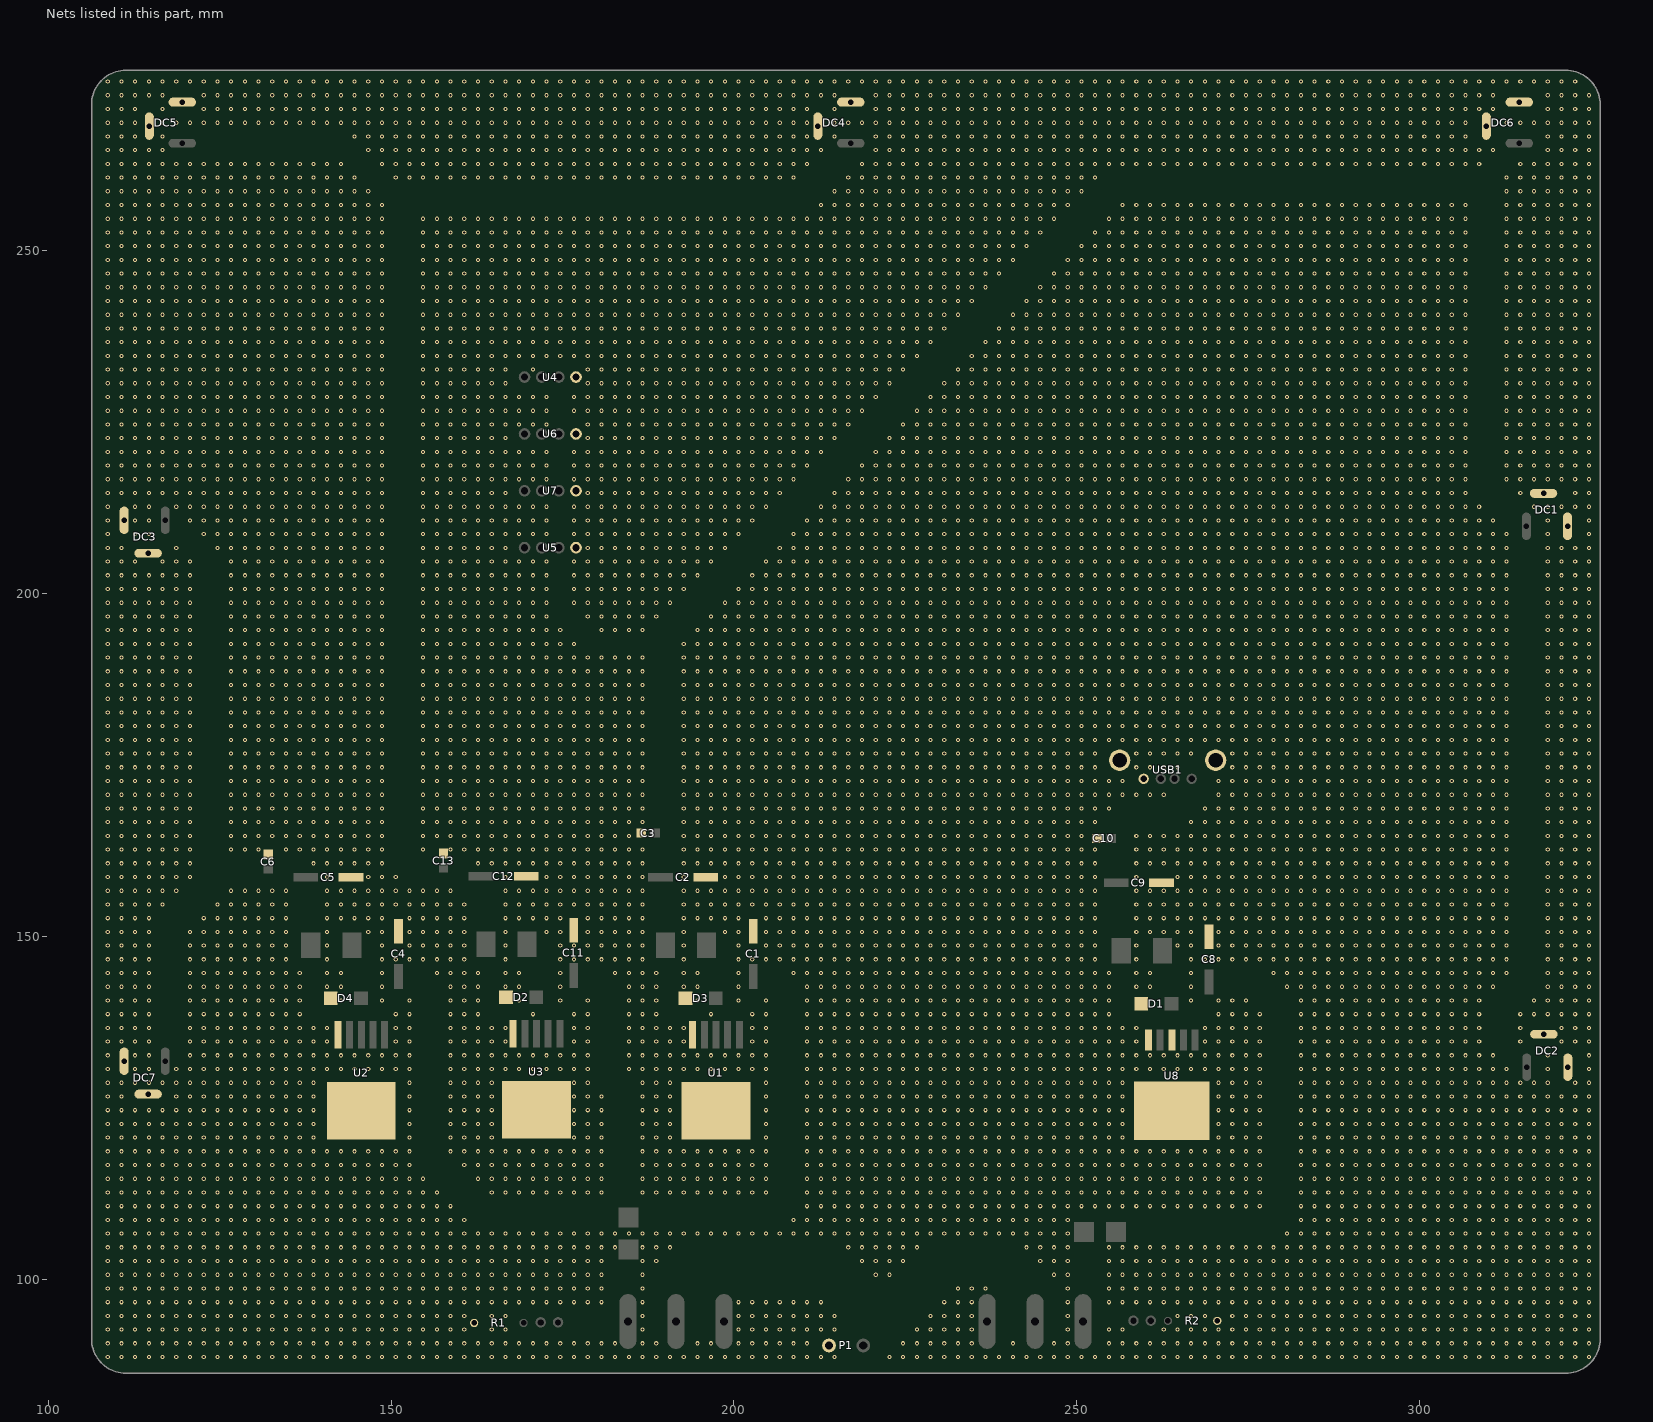
[diagram p0: the nets of this part, all layers, seen from the top]
# Altium PCB MISC49942.pcbdoc (part 3 of 4)
Units mm, origin at the board's own origin, x right, y up, seen from the top; angles counter-clockwise.
Board outline 220 x 190 mm, 2 copper layers (Top Layer, Bottom Layer), stack 1.58 mm thick; 45 components, 14 nets, 127 pads, 8689 vias.

## Via types
v1: diameter 0.61, hole 0.305, Top Layer to Bottom Layer, 8689 vias

## Nets (pads, with @x,y where several pads share a name; then routed paths per layer and width w, separated by ;. In a path a pad name is that pad's centre, name@x,y a point inside that pad or via, vN(x,y) a via of type N, cw(c..) or ccw(c..) an arc to the next point about the centre after c; other vN are vias at no path point) (continued)
GND: (continued)
  other v1: 270.684,158.669 272.684,158.669 274.684,158.669 276.684,158.669 278.684,158.669 280.684,158.669 282.684,158.669 284.684,158.669 286.684,158.669 288.684,158.669 290.684,158.669 292.684,158.669 294.684,158.669 296.684,158.669 298.684,158.669 300.684,158.669 302.684,158.669 304.684,158.669 306.684,158.669 308.684,158.669 310.684,158.669 312.684,158.669 318.684,158.669 320.684,158.669 322.684,158.669 324.684,158.669 108.684,160.669 110.684,160.669 112.684,160.669 114.684,160.669 116.684,160.669 118.684,160.669 120.684,160.669 138.684,160.669 140.684,160.669 142.684,160.669 144.684,160.669 146.684,160.669 148.684,160.669 162.684,160.669 164.684,160.669 166.684,160.669 168.684,160.669 170.684,160.669 172.684,160.669 174.684,160.669 176.684,160.669 178.684,160.669 180.684,160.669 182.684,160.669 184.684,160.669 186.684,160.669 192.684,160.669 194.684,160.669 196.684,160.669 198.684,160.669 200.684,160.669 202.684,160.669 204.684,160.669 206.684,160.669 208.684,160.669 210.684,160.669 212.684,160.669 214.684,160.669 216.684,160.669 218.684,160.669 220.684,160.669 222.684,160.669 224.684,160.669 226.684,160.669 228.684,160.669 230.684,160.669 232.684,160.669 234.684,160.669 236.684,160.669 238.684,160.669 240.684,160.669 242.684,160.669 244.684,160.669 246.684,160.669 248.684,160.669 250.684,160.669 252.684,160.669 258.684,160.669 260.684,160.669 262.684,160.669 264.684,160.669 266.684,160.669 268.684,160.669 270.684,160.669 272.684,160.669 274.684,160.669 276.684,160.669 278.684,160.669 280.684,160.669 282.684,160.669 284.684,160.669 286.684,160.669 288.684,160.669 290.684,160.669 292.684,160.669 294.684,160.669 296.684,160.669 298.684,160.669 300.684,160.669 302.684,160.669 304.684,160.669 306.684,160.669 308.684,160.669 310.684,160.669 312.684,160.669 318.684,160.669 320.684,160.669 322.684,160.669 324.684,160.669 108.684,162.669 110.684,162.669 112.684,162.669 114.684,162.669 116.684,162.669 118.684,162.669 120.684,162.669 126.684,162.669 128.684,162.669 130.684,162.669 134.684,162.669 136.684,162.669 138.684,162.669 140.684,162.669 142.684,162.669 144.684,162.669 146.684,162.669 148.684,162.669 154.684,162.669 158.684,162.669 160.684,162.669 162.684,162.669 164.684,162.669 166.684,162.669 168.684,162.669 170.684,162.669 172.684,162.669 174.684,162.669 176.684,162.669 178.684,162.669 180.684,162.669 182.684,162.669 184.684,162.669 186.684,162.669 192.684,162.669 194.684,162.669 196.684,162.669 198.684,162.669 200.684,162.669 202.684,162.669 204.684,162.669 206.684,162.669 208.684,162.669 210.684,162.669 212.684,162.669 214.684,162.669 216.684,162.669 218.684,162.669 220.684,162.669 222.684,162.669 224.684,162.669 226.684,162.669 228.684,162.669 230.684,162.669 232.684,162.669 234.684,162.669 236.684,162.669 238.684,162.669 240.684,162.669 242.684,162.669 244.684,162.669 246.684,162.669 248.684,162.669 250.684,162.669 252.684,162.669 258.684,162.669 260.684,162.669 262.684,162.669 264.684,162.669 266.684,162.669 268.684,162.669 270.684,162.669 272.684,162.669 274.684,162.669 276.684,162.669 278.684,162.669 280.684,162.669 282.684,162.669 284.684,162.669 286.684,162.669 288.684,162.669 290.684,162.669 292.684,162.669 294.684,162.669 296.684,162.669 298.684,162.669 300.684,162.669 302.684,162.669 304.684,162.669 306.684,162.669 308.684,162.669 310.684,162.669 312.684,162.669 318.684,162.669 320.684,162.669 322.684,162.669 324.684,162.669 108.684,164.669 110.684,164.669 112.684,164.669 114.684,164.669 116.684,164.669 118.684,164.669 120.684,164.669 126.684,164.669 128.684,164.669 130.684,164.669 132.684,164.669 134.684,164.669 136.684,164.669 138.684,164.669 140.684,164.669 142.684,164.669 144.684,164.669 146.684,164.669 148.684,164.669 154.684,164.669 156.684,164.669 158.684,164.669 160.684,164.669 162.684,164.669 164.684,164.669 166.684,164.669 168.684,164.669 170.684,164.669 172.684,164.669 174.684,164.669 176.684,164.669 178.684,164.669 180.684,164.669 182.684,164.669 184.684,164.669 192.684,164.669 194.684,164.669 196.684,164.669 198.684,164.669 200.684,164.669 202.684,164.669 204.684,164.669 206.684,164.669 208.684,164.669 210.684,164.669 212.684,164.669 214.684,164.669 216.684,164.669 218.684,164.669 220.684,164.669 222.684,164.669 224.684,164.669 226.684,164.669 228.684,164.669 230.684,164.669 232.684,164.669 234.684,164.669 236.684,164.669 238.684,164.669 240.684,164.669 242.684,164.669 244.684,164.669 246.684,164.669 248.684,164.669 250.684,164.669 258.684,164.669 260.684,164.669 262.684,164.669 264.684,164.669 266.684,164.669 268.684,164.669 270.684,164.669 272.684,164.669 274.684,164.669 276.684,164.669 278.684,164.669 280.684,164.669 282.684,164.669 284.684,164.669 286.684,164.669 288.684,164.669 290.684,164.669 292.684,164.669 294.684,164.669 296.684,164.669 298.684,164.669 300.684,164.669 302.684,164.669 304.684,164.669 306.684,164.669 308.684,164.669 310.684,164.669 312.684,164.669 318.684,164.669 320.684,164.669 322.684,164.669 324.684,164.669 108.684,166.669 110.684,166.669 112.684,166.669 114.684,166.669 116.684,166.669 118.684,166.669 120.684,166.669 126.684,166.669 128.684,166.669 130.684,166.669 132.684,166.669 134.684,166.669 136.684,166.669 138.684,166.669 140.684,166.669 142.684,166.669 144.684,166.669 146.684,166.669 148.684,166.669 154.684,166.669 156.684,166.669 158.684,166.669 160.684,166.669 162.684,166.669 164.684,166.669 166.684,166.669 168.684,166.669 170.684,166.669 172.684,166.669 174.684,166.669 176.684,166.669 178.684,166.669 180.684,166.669 182.684,166.669 184.684,166.669 186.684,166.669 192.684,166.669 194.684,166.669 196.684,166.669 198.684,166.669 200.684,166.669 202.684,166.669 204.684,166.669 206.684,166.669 208.684,166.669 210.684,166.669 212.684,166.669 214.684,166.669 216.684,166.669 218.684,166.669 220.684,166.669 222.684,166.669 224.684,166.669 226.684,166.669 228.684,166.669 230.684,166.669 232.684,166.669 234.684,166.669 236.684,166.669 238.684,166.669 240.684,166.669 242.684,166.669 244.684,166.669 246.684,166.669 248.684,166.669 250.684,166.669 252.684,166.669 266.684,166.669 268.684,166.669 270.684,166.669 272.684,166.669 274.684,166.669 276.684,166.669 278.684,166.669 280.684,166.669 282.684,166.669 284.684,166.669 286.684,166.669 288.684,166.669 290.684,166.669 292.684,166.669 294.684,166.669 296.684,166.669 298.684,166.669 300.684,166.669 302.684,166.669 304.684,166.669 306.684,166.669 308.684,166.669 310.684,166.669 312.684,166.669 318.684,166.669 320.684,166.669 322.684,166.669 324.684,166.669 108.684,168.669 110.684,168.669 112.684,168.669 114.684,168.669 116.684,168.669 118.684,168.669 120.684,168.669 126.684,168.669 128.684,168.669 130.684,168.669 132.684,168.669 134.684,168.669 136.684,168.669 138.684,168.669 140.684,168.669 142.684,168.669 144.684,168.669 146.684,168.669 148.684,168.669 154.684,168.669 156.684,168.669 158.684,168.669 160.684,168.669 162.684,168.669 164.684,168.669 166.684,168.669 168.684,168.669 170.684,168.669 172.684,168.669 174.684,168.669 176.684,168.669 178.684,168.669 180.684,168.669 182.684,168.669 184.684,168.669 186.684,168.669 192.684,168.669 194.684,168.669 196.684,168.669 198.684,168.669 200.684,168.669 202.684,168.669 204.684,168.669 206.684,168.669 208.684,168.669 210.684,168.669 212.684,168.669 214.684,168.669 216.684,168.669 218.684,168.669 220.684,168.669 222.684,168.669 224.684,168.669 226.684,168.669 228.684,168.669 230.684,168.669 232.684,168.669 234.684,168.669 236.684,168.669 238.684,168.669 240.684,168.669 242.684,168.669 244.684,168.669 246.684,168.669 248.684,168.669 250.684,168.669 252.684,168.669 254.684,168.669 268.684,168.669 270.684,168.669 272.684,168.669 274.684,168.669 276.684,168.669 278.684,168.669 280.684,168.669 282.684,168.669 284.684,168.669 286.684,168.669 288.684,168.669 290.684,168.669 292.684,168.669 294.684,168.669 296.684,168.669 298.684,168.669 300.684,168.669 302.684,168.669 304.684,168.669 306.684,168.669 308.684,168.669 310.684,168.669 312.684,168.669 318.684,168.669 320.684,168.669 322.684,168.669 324.684,168.669 108.684,170.669 110.684,170.669 112.684,170.669 114.684,170.669 116.684,170.669 118.684,170.669 120.684,170.669 126.684,170.669 128.684,170.669 130.684,170.669 132.684,170.669 134.684,170.669 136.684,170.669 138.684,170.669 140.684,170.669 142.684,170.669 144.684,170.669 146.684,170.669 148.684,170.669 154.684,170.669 156.684,170.669 158.684,170.669 160.684,170.669 162.684,170.669 164.684,170.669 166.684,170.669 168.684,170.669 170.684,170.669 172.684,170.669 174.684,170.669 176.684,170.669 178.684,170.669 180.684,170.669 182.684,170.669 184.684,170.669 186.684,170.669 192.684,170.669 194.684,170.669 196.684,170.669 198.684,170.669 200.684,170.669 202.684,170.669 204.684,170.669 206.684,170.669 208.684,170.669 210.684,170.669 212.684,170.669 214.684,170.669 216.684,170.669 218.684,170.669 220.684,170.669 222.684,170.669 224.684,170.669 226.684,170.669 228.684,170.669 230.684,170.669 232.684,170.669 234.684,170.669 236.684,170.669 238.684,170.669 240.684,170.669 242.684,170.669 244.684,170.669 246.684,170.669 248.684,170.669 250.684,170.669 252.684,170.669 254.684,170.669 256.684,170.669 258.684,170.669 260.684,170.669 262.684,170.669 270.684,170.669 272.684,170.669 274.684,170.669 276.684,170.669 278.684,170.669 280.684,170.669 282.684,170.669 284.684,170.669 286.684,170.669 288.684,170.669 290.684,170.669 292.684,170.669 294.684,170.669 296.684,170.669 298.684,170.669 300.684,170.669 302.684,170.669 304.684,170.669 306.684,170.669 308.684,170.669 310.684,170.669 312.684,170.669 318.684,170.669 320.684,170.669 322.684,170.669 324.684,170.669 108.684,172.669 110.684,172.669 112.684,172.669 114.684,172.669 116.684,172.669 118.684,172.669 120.684,172.669 126.684,172.669 128.684,172.669 130.684,172.669 132.684,172.669 134.684,172.669 136.684,172.669 138.684,172.669 140.684,172.669 142.684,172.669 144.684,172.669 146.684,172.669 148.684,172.669 154.684,172.669 156.684,172.669 158.684,172.669 160.684,172.669 162.684,172.669 164.684,172.669 166.684,172.669 168.684,172.669 170.684,172.669 172.684,172.669 174.684,172.669 176.684,172.669 178.684,172.669 180.684,172.669 182.684,172.669 184.684,172.669 186.684,172.669 192.684,172.669 194.684,172.669 196.684,172.669 198.684,172.669 200.684,172.669 202.684,172.669 204.684,172.669 206.684,172.669 208.684,172.669 210.684,172.669 212.684,172.669 214.684,172.669 216.684,172.669 218.684,172.669 220.684,172.669 222.684,172.669 224.684,172.669 226.684,172.669 228.684,172.669 230.684,172.669 232.684,172.669 234.684,172.669 236.684,172.669 238.684,172.669 240.684,172.669 242.684,172.669 244.684,172.669 246.684,172.669 248.684,172.669 250.684,172.669 252.684,172.669 254.684,172.669 256.684,172.669 270.684,172.669 272.684,172.669 274.684,172.669 276.684,172.669 278.684,172.669 280.684,172.669 282.684,172.669 284.684,172.669 286.684,172.669 288.684,172.669 290.684,172.669 292.684,172.669 294.684,172.669 296.684,172.669 298.684,172.669 300.684,172.669 302.684,172.669 304.684,172.669 306.684,172.669 308.684,172.669 310.684,172.669 312.684,172.669 318.684,172.669 320.684,172.669 322.684,172.669 324.684,172.669 108.684,174.669 110.684,174.669 112.684,174.669 114.684,174.669 116.684,174.669 118.684,174.669 120.684,174.669 126.684,174.669 128.684,174.669 130.684,174.669 132.684,174.669 134.684,174.669 136.684,174.669 138.684,174.669 140.684,174.669 142.684,174.669 144.684,174.669 146.684,174.669 148.684,174.669 154.684,174.669 156.684,174.669 158.684,174.669 160.684,174.669 162.684,174.669 164.684,174.669 166.684,174.669 168.684,174.669 170.684,174.669 172.684,174.669 174.684,174.669 176.684,174.669 178.684,174.669 180.684,174.669 182.684,174.669 184.684,174.669 186.684,174.669 192.684,174.669 194.684,174.669 196.684,174.669 198.684,174.669 200.684,174.669 202.684,174.669 204.684,174.669 206.684,174.669 208.684,174.669 210.684,174.669 212.684,174.669 214.684,174.669 216.684,174.669 218.684,174.669 220.684,174.669 222.684,174.669 224.684,174.669 226.684,174.669 228.684,174.669 230.684,174.669 232.684,174.669 234.684,174.669 236.684,174.669 238.684,174.669 240.684,174.669 242.684,174.669 244.684,174.669 246.684,174.669 248.684,174.669 250.684,174.669 252.684,174.669 258.684,174.669 260.684,174.669 262.684,174.669 264.684,174.669 272.684,174.669 274.684,174.669 276.684,174.669 278.684,174.669 280.684,174.669 282.684,174.669 284.684,174.669 286.684,174.669 288.684,174.669 290.684,174.669 292.684,174.669 294.684,174.669 296.684,174.669 298.684,174.669 300.684,174.669 302.684,174.669 304.684,174.669 306.684,174.669 308.684,174.669 310.684,174.669 312.684,174.669 318.684,174.669 320.684,174.669 322.684,174.669 324.684,174.669 108.684,176.669 110.684,176.669 112.684,176.669 114.684,176.669 116.684,176.669 118.684,176.669 120.684,176.669 126.684,176.669 128.684,176.669 130.684,176.669 132.684,176.669 134.684,176.669 136.684,176.669 138.684,176.669 140.684,176.669 142.684,176.669 144.684,176.669 146.684,176.669 148.684,176.669 154.684,176.669 156.684,176.669 158.684,176.669 160.684,176.669 162.684,176.669 164.684,176.669 166.684,176.669 168.684,176.669 170.684,176.669 172.684,176.669 174.684,176.669 176.684,176.669 178.684,176.669 180.684,176.669 182.684,176.669 184.684,176.669 186.684,176.669 192.684,176.669 194.684,176.669 196.684,176.669 198.684,176.669 200.684,176.669 202.684,176.669 204.684,176.669 206.684,176.669 208.684,176.669 210.684,176.669 212.684,176.669 214.684,176.669 216.684,176.669 218.684,176.669 220.684,176.669 222.684,176.669 224.684,176.669 226.684,176.669 228.684,176.669 230.684,176.669 232.684,176.669 234.684,176.669 236.684,176.669 238.684,176.669 240.684,176.669 242.684,176.669 244.684,176.669 246.684,176.669 248.684,176.669 250.684,176.669 252.684,176.669 258.684,176.669 260.684,176.669 262.684,176.669 264.684,176.669 266.684,176.669 272.684,176.669 274.684,176.669 276.684,176.669 278.684,176.669 280.684,176.669 282.684,176.669 284.684,176.669 286.684,176.669 288.684,176.669 290.684,176.669 292.684,176.669 294.684,176.669 296.684,176.669 298.684,176.669 300.684,176.669 302.684,176.669 304.684,176.669 306.684,176.669 308.684,176.669 310.684,176.669 312.684,176.669 318.684,176.669 320.684,176.669 322.684,176.669 324.684,176.669 108.684,178.669 110.684,178.669 112.684,178.669 114.684,178.669 116.684,178.669 118.684,178.669 120.684,178.669 126.684,178.669 128.684,178.669 130.684,178.669 132.684,178.669 134.684,178.669 136.684,178.669 138.684,178.669 140.684,178.669 142.684,178.669 144.684,178.669 146.684,178.669 148.684,178.669 154.684,178.669 156.684,178.669 158.684,178.669 160.684,178.669 162.684,178.669 164.684,178.669 166.684,178.669 168.684,178.669 170.684,178.669 172.684,178.669 174.684,178.669 176.684,178.669 178.684,178.669 180.684,178.669 182.684,178.669 184.684,178.669 186.684,178.669 192.684,178.669 194.684,178.669 196.684,178.669 198.684,178.669 200.684,178.669 202.684,178.669 204.684,178.669 206.684,178.669 208.684,178.669 210.684,178.669 212.684,178.669 214.684,178.669 216.684,178.669 218.684,178.669 220.684,178.669 222.684,178.669 224.684,178.669 226.684,178.669 228.684,178.669 230.684,178.669 232.684,178.669 234.684,178.669 236.684,178.669 238.684,178.669 240.684,178.669 242.684,178.669 244.684,178.669 246.684,178.669 248.684,178.669 250.684,178.669 252.684,178.669 254.684,178.669 256.684,178.669 258.684,178.669 260.684,178.669 262.684,178.669 264.684,178.669 266.684,178.669 268.684,178.669 270.684,178.669 272.684,178.669 274.684,178.669 276.684,178.669 278.684,178.669 280.684,178.669 282.684,178.669 284.684,178.669 286.684,178.669 288.684,178.669 290.684,178.669 292.684,178.669 294.684,178.669 296.684,178.669 298.684,178.669 300.684,178.669 302.684,178.669 304.684,178.669 306.684,178.669 308.684,178.669 310.684,178.669 312.684,178.669 318.684,178.669 320.684,178.669 322.684,178.669 324.684,178.669 108.684,180.669 110.684,180.669 112.684,180.669 114.684,180.669 116.684,180.669 118.684,180.669 120.684,180.669 126.684,180.669 128.684,180.669 130.684,180.669 132.684,180.669 134.684,180.669 136.684,180.669 138.684,180.669 140.684,180.669 142.684,180.669 144.684,180.669 146.684,180.669 148.684,180.669 154.684,180.669 156.684,180.669 158.684,180.669 160.684,180.669 162.684,180.669 164.684,180.669 166.684,180.669 168.684,180.669 170.684,180.669 172.684,180.669 174.684,180.669 176.684,180.669 178.684,180.669 180.684,180.669 182.684,180.669 184.684,180.669 186.684,180.669 192.684,180.669 194.684,180.669 196.684,180.669 198.684,180.669 200.684,180.669 202.684,180.669 204.684,180.669 206.684,180.669 208.684,180.669 210.684,180.669 212.684,180.669 214.684,180.669 216.684,180.669 218.684,180.669 220.684,180.669 222.684,180.669 224.684,180.669 226.684,180.669 228.684,180.669 230.684,180.669 232.684,180.669 234.684,180.669 236.684,180.669 238.684,180.669 240.684,180.669 242.684,180.669 244.684,180.669 246.684,180.669 248.684,180.669 250.684,180.669 252.684,180.669 254.684,180.669 256.684,180.669 258.684,180.669 260.684,180.669 262.684,180.669 264.684,180.669 266.684,180.669 268.684,180.669 270.684,180.669 272.684,180.669 274.684,180.669 276.684,180.669 278.684,180.669 280.684,180.669 282.684,180.669 284.684,180.669 286.684,180.669 288.684,180.669 290.684,180.669 292.684,180.669 294.684,180.669 296.684,180.669 298.684,180.669 300.684,180.669 302.684,180.669 304.684,180.669 306.684,180.669 308.684,180.669 310.684,180.669 312.684,180.669 318.684,180.669 320.684,180.669 322.684,180.669 324.684,180.669 108.684,182.669 110.684,182.669 112.684,182.669 114.684,182.669 116.684,182.669 118.684,182.669 120.684,182.669 126.684,182.669 128.684,182.669 130.684,182.669 132.684,182.669 134.684,182.669 136.684,182.669 138.684,182.669 140.684,182.669 142.684,182.669 144.684,182.669 146.684,182.669 148.684,182.669 154.684,182.669 156.684,182.669 158.684,182.669 160.684,182.669 162.684,182.669 164.684,182.669 166.684,182.669 168.684,182.669 170.684,182.669 172.684,182.669 174.684,182.669 176.684,182.669 178.684,182.669 180.684,182.669 182.684,182.669 184.684,182.669 186.684,182.669 192.684,182.669 194.684,182.669 196.684,182.669 198.684,182.669 200.684,182.669 202.684,182.669 204.684,182.669 206.684,182.669 208.684,182.669 210.684,182.669 212.684,182.669 214.684,182.669 216.684,182.669 218.684,182.669 220.684,182.669 222.684,182.669 224.684,182.669 226.684,182.669 228.684,182.669 230.684,182.669 232.684,182.669 234.684,182.669 236.684,182.669 238.684,182.669 240.684,182.669 242.684,182.669 244.684,182.669 246.684,182.669 248.684,182.669 250.684,182.669 252.684,182.669 254.684,182.669 256.684,182.669 258.684,182.669 260.684,182.669 262.684,182.669 264.684,182.669 266.684,182.669 268.684,182.669 270.684,182.669 272.684,182.669 274.684,182.669 276.684,182.669 278.684,182.669 280.684,182.669 282.684,182.669 284.684,182.669 286.684,182.669 288.684,182.669 290.684,182.669 292.684,182.669 294.684,182.669 296.684,182.669 298.684,182.669 300.684,182.669 302.684,182.669 304.684,182.669 306.684,182.669 308.684,182.669 310.684,182.669 312.684,182.669 318.684,182.669 320.684,182.669 322.684,182.669 324.684,182.669 108.684,184.669 110.684,184.669 112.684,184.669 114.684,184.669 116.684,184.669 118.684,184.669 120.684,184.669 126.684,184.669 128.684,184.669 130.684,184.669 132.684,184.669 134.684,184.669 136.684,184.669 138.684,184.669 140.684,184.669 142.684,184.669 144.684,184.669 146.684,184.669 148.684,184.669 154.684,184.669 156.684,184.669 158.684,184.669 160.684,184.669 162.684,184.669 164.684,184.669 166.684,184.669 168.684,184.669 170.684,184.669 172.684,184.669 174.684,184.669 176.684,184.669 178.684,184.669 180.684,184.669 182.684,184.669 184.684,184.669 186.684,184.669 192.684,184.669 194.684,184.669 196.684,184.669 198.684,184.669 200.684,184.669 202.684,184.669 204.684,184.669 206.684,184.669 208.684,184.669 210.684,184.669 212.684,184.669 214.684,184.669 216.684,184.669 218.684,184.669 220.684,184.669 222.684,184.669 224.684,184.669 226.684,184.669 228.684,184.669 230.684,184.669 232.684,184.669 234.684,184.669 236.684,184.669 238.684,184.669 240.684,184.669 242.684,184.669 244.684,184.669 246.684,184.669 248.684,184.669 250.684,184.669 252.684,184.669 254.684,184.669 256.684,184.669 258.684,184.669 260.684,184.669 262.684,184.669 264.684,184.669 266.684,184.669 268.684,184.669 270.684,184.669 272.684,184.669 274.684,184.669 276.684,184.669 278.684,184.669 280.684,184.669 282.684,184.669 284.684,184.669 286.684,184.669 288.684,184.669 290.684,184.669 292.684,184.669 294.684,184.669 296.684,184.669 298.684,184.669 300.684,184.669 302.684,184.669 304.684,184.669 306.684,184.669 308.684,184.669 310.684,184.669 312.684,184.669 318.684,184.669 320.684,184.669 322.684,184.669 324.684,184.669 108.684,186.669 110.684,186.669 112.684,186.669 114.684,186.669 116.684,186.669 118.684,186.669 120.684,186.669 126.684,186.669 128.684,186.669 130.684,186.669 132.684,186.669 134.684,186.669 136.684,186.669 138.684,186.669 140.684,186.669 142.684,186.669 144.684,186.669 146.684,186.669 148.684,186.669 154.684,186.669 156.684,186.669 158.684,186.669 160.684,186.669 162.684,186.669 164.684,186.669 166.684,186.669 168.684,186.669 170.684,186.669 172.684,186.669 174.684,186.669 176.684,186.669 178.684,186.669 180.684,186.669 182.684,186.669 184.684,186.669 186.684,186.669 192.684,186.669 194.684,186.669 196.684,186.669 198.684,186.669 200.684,186.669 202.684,186.669 204.684,186.669 206.684,186.669 208.684,186.669 210.684,186.669 212.684,186.669 214.684,186.669 216.684,186.669 218.684,186.669 220.684,186.669 222.684,186.669 224.684,186.669 226.684,186.669 228.684,186.669 230.684,186.669 232.684,186.669 234.684,186.669 236.684,186.669 238.684,186.669 240.684,186.669 242.684,186.669 244.684,186.669 246.684,186.669 248.684,186.669 250.684,186.669 252.684,186.669 254.684,186.669 256.684,186.669 258.684,186.669 260.684,186.669 262.684,186.669 264.684,186.669 266.684,186.669 268.684,186.669 270.684,186.669 272.684,186.669 274.684,186.669 276.684,186.669 278.684,186.669 280.684,186.669 282.684,186.669 284.684,186.669 286.684,186.669 288.684,186.669 290.684,186.669 292.684,186.669 294.684,186.669 296.684,186.669 298.684,186.669 300.684,186.669 302.684,186.669 304.684,186.669 306.684,186.669 308.684,186.669 310.684,186.669 312.684,186.669 318.684,186.669 320.684,186.669 322.684,186.669 324.684,186.669 108.684,188.669 110.684,188.669 112.684,188.669 114.684,188.669 116.684,188.669 118.684,188.669 120.684,188.669 126.684,188.669 128.684,188.669 130.684,188.669 132.684,188.669 134.684,188.669 136.684,188.669 138.684,188.669 140.684,188.669 142.684,188.669 144.684,188.669 146.684,188.669 148.684,188.669 154.684,188.669 156.684,188.669 158.684,188.669 160.684,188.669 162.684,188.669 164.684,188.669 166.684,188.669 168.684,188.669 170.684,188.669 172.684,188.669 174.684,188.669 176.684,188.669 178.684,188.669 180.684,188.669 182.684,188.669 184.684,188.669 186.684,188.669 192.684,188.669 194.684,188.669 196.684,188.669 198.684,188.669 200.684,188.669 202.684,188.669 204.684,188.669 206.684,188.669 208.684,188.669 210.684,188.669 212.684,188.669 214.684,188.669 216.684,188.669 218.684,188.669 220.684,188.669 222.684,188.669 224.684,188.669 226.684,188.669 228.684,188.669 230.684,188.669 232.684,188.669 234.684,188.669 236.684,188.669 238.684,188.669 240.684,188.669 242.684,188.669 244.684,188.669 246.684,188.669 248.684,188.669 250.684,188.669 252.684,188.669 254.684,188.669 256.684,188.669 258.684,188.669 260.684,188.669 262.684,188.669 264.684,188.669 266.684,188.669 268.684,188.669 270.684,188.669 272.684,188.669 274.684,188.669 276.684,188.669 278.684,188.669 280.684,188.669 282.684,188.669 284.684,188.669 286.684,188.669 288.684,188.669 290.684,188.669 292.684,188.669 294.684,188.669 296.684,188.669 298.684,188.669 300.684,188.669 302.684,188.669 304.684,188.669 306.684,188.669 308.684,188.669 310.684,188.669 312.684,188.669 318.684,188.669 320.684,188.669 322.684,188.669 324.684,188.669 108.684,190.669 110.684,190.669 112.684,190.669 114.684,190.669 116.684,190.669 118.684,190.669 120.684,190.669 126.684,190.669 128.684,190.669 130.684,190.669 132.684,190.669 134.684,190.669 136.684,190.669 138.684,190.669 140.684,190.669 142.684,190.669 144.684,190.669 146.684,190.669 148.684,190.669 154.684,190.669 156.684,190.669 158.684,190.669 160.684,190.669 162.684,190.669 164.684,190.669 166.684,190.669 168.684,190.669 170.684,190.669 172.684,190.669 174.684,190.669 176.684,190.669 178.684,190.669 180.684,190.669 182.684,190.669 184.684,190.669 186.684,190.669 192.684,190.669 194.684,190.669 196.684,190.669 198.684,190.669 200.684,190.669 202.684,190.669 204.684,190.669 206.684,190.669 208.684,190.669 210.684,190.669 212.684,190.669 214.684,190.669 216.684,190.669 218.684,190.669 220.684,190.669 222.684,190.669 224.684,190.669 226.684,190.669 228.684,190.669 230.684,190.669 232.684,190.669 234.684,190.669 236.684,190.669 238.684,190.669 240.684,190.669 242.684,190.669 244.684,190.669 246.684,190.669 248.684,190.669 250.684,190.669 252.684,190.669 254.684,190.669 256.684,190.669 258.684,190.669 260.684,190.669 262.684,190.669 264.684,190.669 266.684,190.669 268.684,190.669 270.684,190.669 272.684,190.669 274.684,190.669 276.684,190.669 278.684,190.669 280.684,190.669 282.684,190.669 284.684,190.669 286.684,190.669 288.684,190.669 290.684,190.669 292.684,190.669 294.684,190.669 296.684,190.669 298.684,190.669 300.684,190.669 302.684,190.669 304.684,190.669 306.684,190.669 308.684,190.669 310.684,190.669 312.684,190.669 318.684,190.669 320.684,190.669 322.684,190.669 324.684,190.669 108.684,192.669 110.684,192.669 112.684,192.669 114.684,192.669 116.684,192.669 118.684,192.669 120.684,192.669 126.684,192.669 128.684,192.669 130.684,192.669 132.684,192.669 134.684,192.669 136.684,192.669 138.684,192.669 140.684,192.669 142.684,192.669 144.684,192.669 146.684,192.669 148.684,192.669 154.684,192.669 156.684,192.669 158.684,192.669 160.684,192.669 162.684,192.669 164.684,192.669 166.684,192.669 168.684,192.669 170.684,192.669 172.684,192.669 174.684,192.669 176.684,192.669 192.684,192.669 194.684,192.669 196.684,192.669 198.684,192.669 200.684,192.669 202.684,192.669 204.684,192.669 206.684,192.669 208.684,192.669 210.684,192.669 212.684,192.669 214.684,192.669 216.684,192.669 218.684,192.669 220.684,192.669 222.684,192.669 224.684,192.669 226.684,192.669 228.684,192.669 230.684,192.669 232.684,192.669 234.684,192.669 236.684,192.669 238.684,192.669 240.684,192.669 242.684,192.669 244.684,192.669 246.684,192.669 248.684,192.669 250.684,192.669 252.684,192.669 254.684,192.669 256.684,192.669 258.684,192.669 260.684,192.669 262.684,192.669 264.684,192.669 266.684,192.669 268.684,192.669 270.684,192.669 272.684,192.669 274.684,192.669 276.684,192.669 278.684,192.669 280.684,192.669 282.684,192.669 284.684,192.669 286.684,192.669 288.684,192.669 290.684,192.669 292.684,192.669 294.684,192.669 296.684,192.669 298.684,192.669 300.684,192.669 302.684,192.669 304.684,192.669 306.684,192.669 308.684,192.669 310.684,192.669 312.684,192.669 318.684,192.669 320.684,192.669 322.684,192.669 324.684,192.669 108.684,194.669 110.684,194.669 112.684,194.669 114.684,194.669 116.684,194.669 118.684,194.669 120.684,194.669 126.684,194.669 128.684,194.669 130.684,194.669 132.684,194.669 134.684,194.669 136.684,194.669 138.684,194.669 140.684,194.669 142.684,194.669 144.684,194.669 146.684,194.669 148.684,194.669 154.684,194.669 156.684,194.669 158.684,194.669 160.684,194.669 162.684,194.669 164.684,194.669 166.684,194.669 168.684,194.669 170.684,194.669 172.684,194.669 174.684,194.669 180.684,194.669 182.684,194.669 184.684,194.669 186.684,194.669 194.684,194.669 196.684,194.669 198.684,194.669 200.684,194.669 202.684,194.669 204.684,194.669 206.684,194.669 208.684,194.669 210.684,194.669 212.684,194.669 214.684,194.669 216.684,194.669 218.684,194.669 220.684,194.669 222.684,194.669 224.684,194.669 226.684,194.669 228.684,194.669 230.684,194.669 232.684,194.669 234.684,194.669 236.684,194.669 238.684,194.669 240.684,194.669 242.684,194.669 244.684,194.669 246.684,194.669 248.684,194.669 250.684,194.669 252.684,194.669 254.684,194.669 256.684,194.669 258.684,194.669 260.684,194.669 262.684,194.669 264.684,194.669 266.684,194.669 268.684,194.669 270.684,194.669 272.684,194.669 274.684,194.669 276.684,194.669 278.684,194.669 280.684,194.669 282.684,194.669 284.684,194.669 286.684,194.669 288.684,194.669 290.684,194.669 292.684,194.669 294.684,194.669 296.684,194.669 298.684,194.669 300.684,194.669 302.684,194.669 304.684,194.669 306.684,194.669 308.684,194.669 310.684,194.669 312.684,194.669 318.684,194.669 320.684,194.669 322.684,194.669 324.684,194.669 108.684,196.669 110.684,196.669 112.684,196.669 114.684,196.669 116.684,196.669 118.684,196.669 120.684,196.669 126.684,196.669 128.684,196.669 130.684,196.669 132.684,196.669 134.684,196.669 136.684,196.669 138.684,196.669 140.684,196.669 142.684,196.669 144.684,196.669 146.684,196.669 148.684,196.669 154.684,196.669 156.684,196.669 158.684,196.669 160.684,196.669 162.684,196.669 164.684,196.669 166.684,196.669 168.684,196.669 170.684,196.669 172.684,196.669 178.684,196.669 180.684,196.669 182.684,196.669 184.684,196.669 186.684,196.669 188.684,196.669 196.684,196.669 198.684,196.669 200.684,196.669 202.684,196.669 204.684,196.669 206.684,196.669 208.684,196.669 210.684,196.669 212.684,196.669 214.684,196.669 216.684,196.669 218.684,196.669 220.684,196.669 222.684,196.669 224.684,196.669 226.684,196.669 228.684,196.669 230.684,196.669 232.684,196.669 234.684,196.669 236.684,196.669 238.684,196.669 240.684,196.669 242.684,196.669 244.684,196.669 246.684,196.669 248.684,196.669 250.684,196.669 252.684,196.669 254.684,196.669 256.684,196.669 258.684,196.669 260.684,196.669 262.684,196.669 264.684,196.669 266.684,196.669 268.684,196.669 270.684,196.669 272.684,196.669 274.684,196.669 276.684,196.669 278.684,196.669 280.684,196.669 282.684,196.669 284.684,196.669 286.684,196.669 288.684,196.669 290.684,196.669 292.684,196.669 294.684,196.669 296.684,196.669 298.684,196.669 300.684,196.669 302.684,196.669 304.684,196.669 306.684,196.669 308.684,196.669 310.684,196.669 312.684,196.669 318.684,196.669 320.684,196.669 322.684,196.669 324.684,196.669 108.684,198.669 110.684,198.669 112.684,198.669 114.684,198.669 116.684,198.669 118.684,198.669 120.684,198.669 126.684,198.669 128.684,198.669 130.684,198.669 132.684,198.669 134.684,198.669 136.684,198.669 138.684,198.669 140.684,198.669 142.684,198.669 144.684,198.669 146.684,198.669 148.684,198.669 154.684,198.669 156.684,198.669 158.684,198.669 160.684,198.669 162.684,198.669 164.684,198.669 166.684,198.669 168.684,198.669 170.684,198.669 172.684,198.669 176.684,198.669 178.684,198.669 180.684,198.669 182.684,198.669 184.684,198.669 186.684,198.669 188.684,198.669 190.684,198.669 198.684,198.669 200.684,198.669 202.684,198.669 204.684,198.669 206.684,198.669 208.684,198.669 210.684,198.669 212.684,198.669 214.684,198.669 216.684,198.669 218.684,198.669 220.684,198.669 222.684,198.669 224.684,198.669 226.684,198.669 228.684,198.669 230.684,198.669 232.684,198.669 234.684,198.669 236.684,198.669 238.684,198.669 240.684,198.669 242.684,198.669 244.684,198.669 246.684,198.669 248.684,198.669 250.684,198.669 252.684,198.669 254.684,198.669 256.684,198.669 258.684,198.669 260.684,198.669 262.684,198.669 264.684,198.669 266.684,198.669 268.684,198.669 270.684,198.669 272.684,198.669 274.684,198.669 276.684,198.669 278.684,198.669 280.684,198.669 282.684,198.669 284.684,198.669 286.684,198.669 288.684,198.669 290.684,198.669 292.684,198.669 294.684,198.669 296.684,198.669 298.684,198.669 300.684,198.669 302.684,198.669 304.684,198.669 306.684,198.669 308.684,198.669 310.684,198.669 312.684,198.669 318.684,198.669 320.684,198.669 322.684,198.669 324.684,198.669 108.684,200.669 110.684,200.669 112.684,200.669 114.684,200.669 116.684,200.669 118.684,200.669 120.684,200.669 126.684,200.669 128.684,200.669 130.684,200.669 132.684,200.669 134.684,200.669 136.684,200.669 138.684,200.669 140.684,200.669 142.684,200.669 144.684,200.669 146.684,200.669 148.684,200.669 154.684,200.669 156.684,200.669 158.684,200.669 160.684,200.669 162.684,200.669 164.684,200.669 166.684,200.669 168.684,200.669 170.684,200.669 172.684,200.669 176.684,200.669 178.684,200.669 180.684,200.669 182.684,200.669 184.684,200.669 186.684,200.669 188.684,200.669 190.684,200.669 192.684,200.669 200.684,200.669 202.684,200.669 204.684,200.669 206.684,200.669 208.684,200.669 210.684,200.669 212.684,200.669 214.684,200.669 216.684,200.669 218.684,200.669 220.684,200.669 222.684,200.669 224.684,200.669 226.684,200.669 228.684,200.669 230.684,200.669 232.684,200.669 234.684,200.669 236.684,200.669 238.684,200.669 240.684,200.669 242.684,200.669 244.684,200.669 246.684,200.669 248.684,200.669 250.684,200.669 252.684,200.669 254.684,200.669 256.684,200.669 258.684,200.669 260.684,200.669 262.684,200.669 264.684,200.669 266.684,200.669 268.684,200.669 270.684,200.669 272.684,200.669 274.684,200.669 276.684,200.669 278.684,200.669 280.684,200.669 282.684,200.669 284.684,200.669 286.684,200.669 288.684,200.669 290.684,200.669 292.684,200.669 294.684,200.669 296.684,200.669 298.684,200.669 300.684,200.669 302.684,200.669 304.684,200.669 306.684,200.669 308.684,200.669 310.684,200.669 312.684,200.669 318.684,200.669 320.684,200.669 322.684,200.669 324.684,200.669 108.684,202.669 110.684,202.669 112.684,202.669 114.684,202.669 116.684,202.669 118.684,202.669 120.684,202.669 126.684,202.669 128.684,202.669 130.684,202.669 132.684,202.669 134.684,202.669 136.684,202.669 138.684,202.669 140.684,202.669 142.684,202.669 144.684,202.669 146.684,202.669 148.684,202.669 154.684,202.669 156.684,202.669 158.684,202.669 160.684,202.669 162.684,202.669 164.684,202.669 166.684,202.669 168.684,202.669 170.684,202.669 172.684,202.669 176.684,202.669 178.684,202.669 180.684,202.669 182.684,202.669 184.684,202.669 186.684,202.669 188.684,202.669 190.684,202.669 192.684,202.669 194.684,202.669 202.684,202.669 204.684,202.669 206.684,202.669 208.684,202.669 210.684,202.669 212.684,202.669 214.684,202.669 216.684,202.669 218.684,202.669 220.684,202.669 222.684,202.669 224.684,202.669 226.684,202.669 228.684,202.669 230.684,202.669 232.684,202.669 234.684,202.669 236.684,202.669 238.684,202.669 240.684,202.669 242.684,202.669 244.684,202.669 246.684,202.669 248.684,202.669 250.684,202.669 252.684,202.669 254.684,202.669 256.684,202.669 258.684,202.669 260.684,202.669 262.684,202.669 264.684,202.669 266.684,202.669 268.684,202.669 270.684,202.669 272.684,202.669 274.684,202.669 276.684,202.669 278.684,202.669 280.684,202.669 282.684,202.669 284.684,202.669 286.684,202.669 288.684,202.669 290.684,202.669 292.684,202.669 294.684,202.669 296.684,202.669 298.684,202.669 300.684,202.669 302.684,202.669 304.684,202.669 306.684,202.669 308.684,202.669 310.684,202.669 312.684,202.669 318.684,202.669 320.684,202.669 322.684,202.669 324.684,202.669 108.684,204.669 110.684,204.669 112.684,204.669 116.684,204.669 118.684,204.669 120.684,204.669 126.684,204.669 128.684,204.669 130.684,204.669 132.684,204.669 134.684,204.669 136.684,204.669 138.684,204.669 140.684,204.669 142.684,204.669 144.684,204.669 146.684,204.669 148.684,204.669 154.684,204.669 156.684,204.669 158.684,204.669 160.684,204.669 162.684,204.669 164.684,204.669 166.684,204.669 168.684,204.669 170.684,204.669 172.684,204.669 176.684,204.669 178.684,204.669 180.684,204.669 182.684,204.669 184.684,204.669 186.684,204.669 188.684,204.669 190.684,204.669 192.684,204.669 194.684,204.669 196.684,204.669 204.684,204.669 206.684,204.669 208.684,204.669 210.684,204.669 212.684,204.669 214.684,204.669 216.684,204.669 218.684,204.669 220.684,204.669 222.684,204.669 224.684,204.669 226.684,204.669 228.684,204.669 230.684,204.669 232.684,204.669 234.684,204.669 236.684,204.669 238.684,204.669 240.684,204.669 242.684,204.669 244.684,204.669 246.684,204.669 248.684,204.669 250.684,204.669 252.684,204.669 254.684,204.669 256.684,204.669 258.684,204.669 260.684,204.669 262.684,204.669 264.684,204.669 266.684,204.669 268.684,204.669 270.684,204.669 272.684,204.669 274.684,204.669 276.684,204.669 278.684,204.669 280.684,204.669 282.684,204.669 284.684,204.669 286.684,204.669 288.684,204.669 290.684,204.669 292.684,204.669 294.684,204.669 296.684,204.669 298.684,204.669 300.684,204.669 302.684,204.669 304.684,204.669 306.684,204.669 308.684,204.669 310.684,204.669 312.684,204.669 318.684,204.669 320.684,204.669 322.684,204.669 324.684,204.669 108.684,206.669 110.684,206.669 118.684,206.669 124.684,206.669 126.684,206.669 128.684,206.669 130.684,206.669 132.684,206.669 134.684,206.669 136.684,206.669 138.684,206.669 140.684,206.669 142.684,206.669 144.684,206.669 146.684,206.669 148.684,206.669 154.684,206.669 156.684,206.669 158.684,206.669 160.684,206.669 162.684,206.669 164.684,206.669 166.684,206.669 178.684,206.669 180.684,206.669 182.684,206.669 184.684,206.669 186.684,206.669 188.684,206.669 190.684,206.669 192.684,206.669 194.684,206.669 196.684,206.669 198.684,206.669 206.684,206.669 208.684,206.669 210.684,206.669 212.684,206.669 214.684,206.669 216.684,206.669 218.684,206.669 220.684,206.669 222.684,206.669 224.684,206.669 226.684,206.669 228.684,206.669 230.684,206.669 232.684,206.669 234.684,206.669 236.684,206.669 238.684,206.669 240.684,206.669 242.684,206.669 244.684,206.669 246.684,206.669 248.684,206.669 250.684,206.669 252.684,206.669 254.684,206.669 256.684,206.669 258.684,206.669 260.684,206.669 262.684,206.669 264.684,206.669 266.684,206.669 268.684,206.669 270.684,206.669 272.684,206.669 274.684,206.669 276.684,206.669 278.684,206.669 280.684,206.669 282.684,206.669 284.684,206.669 286.684,206.669 288.684,206.669 290.684,206.669 292.684,206.669 294.684,206.669 296.684,206.669 298.684,206.669 300.684,206.669 302.684,206.669 304.684,206.669 306.684,206.669 308.684,206.669 310.684,206.669 312.684,206.669 318.684,206.669 320.684,206.669 322.684,206.669 324.684,206.669 108.684,208.669 112.684,208.669 114.684,208.669 122.684,208.669 124.684,208.669 126.684,208.669 128.684,208.669 130.684,208.669 132.684,208.669 134.684,208.669 136.684,208.669 138.684,208.669 140.684,208.669 142.684,208.669 144.684,208.669 146.684,208.669 148.684,208.669 154.684,208.669 156.684,208.669 158.684,208.669 160.684,208.669 162.684,208.669 164.684,208.669 166.684,208.669 168.684,208.669 170.684,208.669 172.684,208.669 176.684,208.669 178.684,208.669 180.684,208.669 182.684,208.669 184.684,208.669 186.684,208.669 188.684,208.669 190.684,208.669 192.684,208.669 194.684,208.669 196.684,208.669 198.684,208.669 200.684,208.669 208.684,208.669 210.684,208.669 212.684,208.669 214.684,208.669 216.684,208.669 218.684,208.669 220.684,208.669 222.684,208.669 224.684,208.669 226.684,208.669 228.684,208.669 230.684,208.669 232.684,208.669 234.684,208.669 236.684,208.669 238.684,208.669 240.684,208.669 242.684,208.669 244.684,208.669 246.684,208.669 248.684,208.669 250.684,208.669 252.684,208.669 254.684,208.669 256.684,208.669 258.684,208.669 260.684,208.669 262.684,208.669 264.684,208.669 266.684,208.669 268.684,208.669 270.684,208.669 272.684,208.669 274.684,208.669 276.684,208.669 278.684,208.669 280.684,208.669 282.684,208.669 284.684,208.669 286.684,208.669 288.684,208.669 290.684,208.669 292.684,208.669 294.684,208.669 296.684,208.669 298.684,208.669 300.684,208.669 302.684,208.669 304.684,208.669 306.684,208.669 308.684,208.669 310.684,208.669 312.684,208.669 318.684,208.669 324.684,208.669 108.684,210.669 112.684,210.669 114.684,210.669 120.684,210.669 122.684,210.669 124.684,210.669 126.684,210.669 128.684,210.669 130.684,210.669 132.684,210.669 134.684,210.669 136.684,210.669 138.684,210.669 140.684,210.669 142.684,210.669 144.684,210.669 146.684,210.669 148.684,210.669 154.684,210.669 156.684,210.669 158.684,210.669 160.684,210.669 162.684,210.669 164.684,210.669 166.684,210.669 168.684,210.669 170.684,210.669 172.684,210.669 176.684,210.669 178.684,210.669 180.684,210.669 182.684,210.669 184.684,210.669 186.684,210.669 188.684,210.669 190.684,210.669 192.684,210.669 194.684,210.669 196.684,210.669 198.684,210.669 200.684,210.669 202.684,210.669 210.684,210.669 212.684,210.669 214.684,210.669 216.684,210.669 218.684,210.669 220.684,210.669 222.684,210.669 224.684,210.669 226.684,210.669 228.684,210.669 230.684,210.669 232.684,210.669 234.684,210.669 236.684,210.669 238.684,210.669 240.684,210.669 242.684,210.669 244.684,210.669 246.684,210.669 248.684,210.669 250.684,210.669 252.684,210.669 254.684,210.669 256.684,210.669 258.684,210.669 260.684,210.669 262.684,210.669 264.684,210.669 266.684,210.669 268.684,210.669 270.684,210.669 272.684,210.669 274.684,210.669 276.684,210.669 278.684,210.669 280.684,210.669 282.684,210.669 284.684,210.669 286.684,210.669 288.684,210.669 290.684,210.669 292.684,210.669 294.684,210.669 296.684,210.669 298.684,210.669 300.684,210.669 302.684,210.669 304.684,210.669 306.684,210.669 308.684,210.669 310.684,210.669 318.684,210.669 324.684,210.669 108.684,212.669 112.684,212.669 114.684,212.669 118.684,212.669 120.684,212.669 122.684,212.669 124.684,212.669 126.684,212.669 128.684,212.669 130.684,212.669 132.684,212.669 134.684,212.669 136.684,212.669 138.684,212.669 140.684,212.669 142.684,212.669 144.684,212.669 146.684,212.669 148.684,212.669 154.684,212.669 156.684,212.669 158.684,212.669 160.684,212.669 162.684,212.669 164.684,212.669 166.684,212.669 168.684,212.669 170.684,212.669 172.684,212.669 176.684,212.669 178.684,212.669 180.684,212.669 182.684,212.669 184.684,212.669 186.684,212.669 188.684,212.669 190.684,212.669 192.684,212.669 194.684,212.669 196.684,212.669 198.684,212.669 200.684,212.669 202.684,212.669 204.684,212.669 212.684,212.669 214.684,212.669 216.684,212.669 218.684,212.669 220.684,212.669 222.684,212.669 224.684,212.669 226.684,212.669 228.684,212.669 230.684,212.669 232.684,212.669 234.684,212.669 236.684,212.669 238.684,212.669 240.684,212.669 242.684,212.669 244.684,212.669 246.684,212.669 248.684,212.669 250.684,212.669 252.684,212.669 254.684,212.669 256.684,212.669 258.684,212.669 260.684,212.669 262.684,212.669 264.684,212.669 266.684,212.669 268.684,212.669 270.684,212.669 272.684,212.669 274.684,212.669 276.684,212.669 278.684,212.669 280.684,212.669 282.684,212.669 284.684,212.669 286.684,212.669 288.684,212.669 290.684,212.669 292.684,212.669 294.684,212.669 296.684,212.669 298.684,212.669 300.684,212.669 302.684,212.669 304.684,212.669 306.684,212.669 308.684,212.669 316.684,212.669 318.684,212.669 320.684,212.669 322.684,212.669 324.684,212.669 108.684,214.669 110.684,214.669 112.684,214.669 114.684,214.669 116.684,214.669 118.684,214.669 120.684,214.669 122.684,214.669 124.684,214.669 126.684,214.669 128.684,214.669 130.684,214.669 132.684,214.669 134.684,214.669 136.684,214.669 138.684,214.669 140.684,214.669 142.684,214.669 144.684,214.669 146.684,214.669 148.684,214.669 154.684,214.669 156.684,214.669 158.684,214.669 160.684,214.669 162.684,214.669 164.684,214.669 166.684,214.669 178.684,214.669 180.684,214.669 182.684,214.669 184.684,214.669 186.684,214.669 188.684,214.669 190.684,214.669 192.684,214.669 194.684,214.669 196.684,214.669 198.684,214.669 200.684,214.669 202.684,214.669 204.684,214.669 206.684,214.669 214.684,214.669 216.684,214.669 218.684,214.669 220.684,214.669 222.684,214.669 224.684,214.669 226.684,214.669 228.684,214.669 230.684,214.669 232.684,214.669 234.684,214.669 236.684,214.669 238.684,214.669 240.684,214.669 242.684,214.669 244.684,214.669 246.684,214.669 248.684,214.669 250.684,214.669 252.684,214.669 254.684,214.669 256.684,214.669 258.684,214.669 260.684,214.669 262.684,214.669 264.684,214.669 266.684,214.669 268.684,214.669 270.684,214.669 272.684,214.669 274.684,214.669 276.684,214.669 278.684,214.669 280.684,214.669 282.684,214.669 284.684,214.669 286.684,214.669 288.684,214.669 290.684,214.669 292.684,214.669 294.684,214.669 296.684,214.669 298.684,214.669 300.684,214.669 302.684,214.669 304.684,214.669 306.684,214.669 314.684,214.669 322.684,214.669 324.684,214.669 108.684,216.669 110.684,216.669 112.684,216.669 114.684,216.669 116.684,216.669 118.684,216.669 120.684,216.669 122.684,216.669 124.684,216.669 126.684,216.669 128.684,216.669 130.684,216.669 132.684,216.669 134.684,216.669 136.684,216.669 138.684,216.669 140.684,216.669 142.684,216.669 144.684,216.669 146.684,216.669 148.684,216.669 154.684,216.669 156.684,216.669 158.684,216.669 160.684,216.669 162.684,216.669 164.684,216.669 166.684,216.669 168.684,216.669 170.684,216.669 172.684,216.669 176.684,216.669 178.684,216.669 180.684,216.669 182.684,216.669 184.684,216.669 186.684,216.669 188.684,216.669 190.684,216.669 192.684,216.669 194.684,216.669 196.684,216.669 198.684,216.669 200.684,216.669 202.684,216.669 204.684,216.669 206.684,216.669 208.684,216.669 216.684,216.669 218.684,216.669 220.684,216.669 222.684,216.669 224.684,216.669 226.684,216.669 228.684,216.669 230.684,216.669 232.684,216.669 234.684,216.669 236.684,216.669 238.684,216.669 240.684,216.669 242.684,216.669 244.684,216.669 246.684,216.669 248.684,216.669 250.684,216.669 252.684,216.669 254.684,216.669 256.684,216.669 258.684,216.669 260.684,216.669 262.684,216.669 264.684,216.669 266.684,216.669 268.684,216.669 270.684,216.669 272.684,216.669 274.684,216.669 276.684,216.669 278.684,216.669 280.684,216.669 282.684,216.669 284.684,216.669 286.684,216.669 288.684,216.669 290.684,216.669 292.684,216.669 294.684,216.669 296.684,216.669 298.684,216.669 300.684,216.669 302.684,216.669 304.684,216.669 306.684,216.669 312.684,216.669 314.684,216.669 316.684,216.669 318.684,216.669 320.684,216.669 322.684,216.669 324.684,216.669 108.684,218.669 110.684,218.669 112.684,218.669 114.684,218.669 116.684,218.669 118.684,218.669 120.684,218.669 122.684,218.669 124.684,218.669 126.684,218.669 128.684,218.669 130.684,218.669 132.684,218.669 134.684,218.669 136.684,218.669 138.684,218.669 140.684,218.669 142.684,218.669 144.684,218.669 146.684,218.669 148.684,218.669 154.684,218.669 156.684,218.669 158.684,218.669 160.684,218.669 162.684,218.669 164.684,218.669 166.684,218.669 168.684,218.669 170.684,218.669 172.684,218.669 176.684,218.669 178.684,218.669 180.684,218.669 182.684,218.669 184.684,218.669 186.684,218.669 188.684,218.669 190.684,218.669 192.684,218.669 194.684,218.669 196.684,218.669 198.684,218.669 200.684,218.669 202.684,218.669 204.684,218.669 206.684,218.669 208.684,218.669 210.684,218.669 218.684,218.669 220.684,218.669 222.684,218.669 224.684,218.669 226.684,218.669 228.684,218.669 230.684,218.669 232.684,218.669 234.684,218.669 236.684,218.669 238.684,218.669 240.684,218.669 242.684,218.669 244.684,218.669 246.684,218.669 248.684,218.669 250.684,218.669 252.684,218.669 254.684,218.669 256.684,218.669 258.684,218.669 260.684,218.669 262.684,218.669 264.684,218.669 266.684,218.669 268.684,218.669 270.684,218.669 272.684,218.669 274.684,218.669 276.684,218.669 278.684,218.669 280.684,218.669 282.684,218.669 284.684,218.669 286.684,218.669 288.684,218.669 290.684,218.669 292.684,218.669 294.684,218.669 296.684,218.669 298.684,218.669 300.684,218.669 302.684,218.669 304.684,218.669 306.684,218.669 312.684,218.669 314.684,218.669 316.684,218.669 318.684,218.669 320.684,218.669 322.684,218.669 324.684,218.669 108.684,220.669 110.684,220.669 112.684,220.669 114.684,220.669 116.684,220.669 118.684,220.669 120.684,220.669 122.684,220.669 124.684,220.669 126.684,220.669 128.684,220.669 130.684,220.669 132.684,220.669 134.684,220.669 136.684,220.669 138.684,220.669 140.684,220.669 142.684,220.669 144.684,220.669 146.684,220.669 148.684,220.669 154.684,220.669 156.684,220.669 158.684,220.669 160.684,220.669 162.684,220.669 164.684,220.669 166.684,220.669 168.684,220.669 170.684,220.669 172.684,220.669 176.684,220.669 178.684,220.669 180.684,220.669 182.684,220.669 184.684,220.669 186.684,220.669 188.684,220.669 190.684,220.669 192.684,220.669 194.684,220.669 196.684,220.669 198.684,220.669 200.684,220.669 202.684,220.669